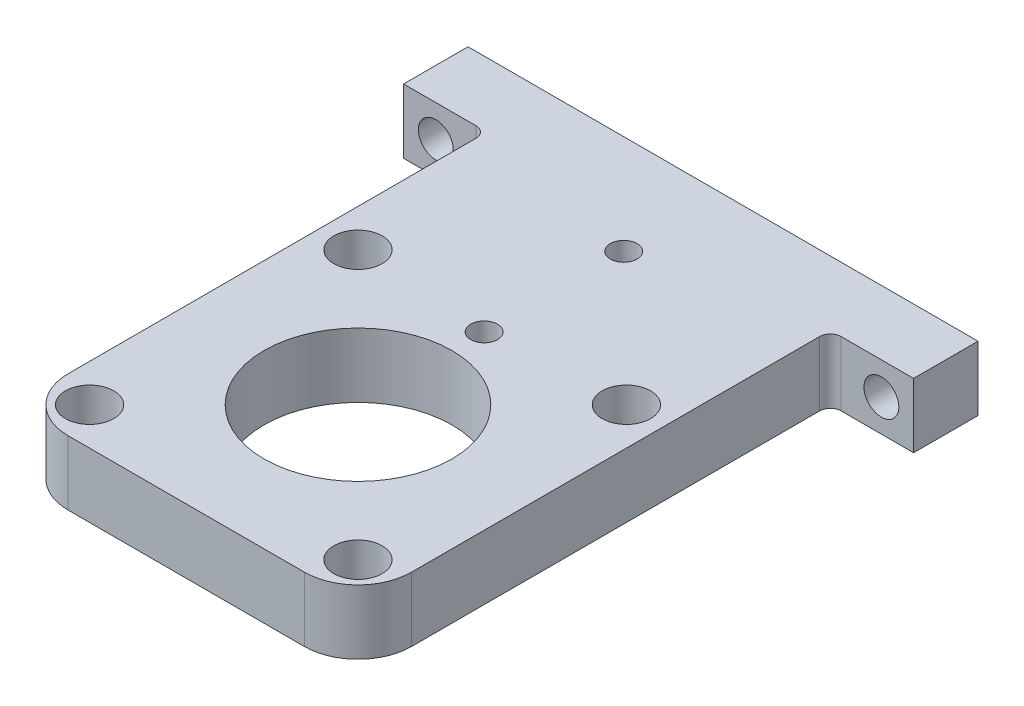
from build123d import *

# Parameters (mm, degrees)
SKETCH_1_W                = 95
SKETCH_1_H                = 100
EXTRUDE_1_DEPTH           = 12
SKETCH_9_W                = 15.5
SKETCH_9_H                = 88
CUT_EXTRUDE_4_DEPTH       = 139.452157802
HOLE_WIZARD_6_5_6_5_1_D   = 6.5
SKETCH_12_R               = 17.5
CUT_EXTRUDE_5_DEPTH       = 139.452157802
FILLET_1_R                = 10
HOLE_WIZARD_5_0_5_1_D     = 5
HOLE_WIZARD_5_0_5_1_DEPTH = 10
HOLE_WIZARD_5_0_5_1_TIP   = 1.502151548
FILLET_2_R                = 2
MM_1_D                    = 9
HOLE_WIZARD_M6_1_D        = 5
HOLE_WIZARD_M6_2_D        = 5


with BuildPart() as part:
    # 草图1 → 凸台-拉伸1 (new body)
    with BuildSketch(Plane(origin=(0, 0, 0), x_dir=(1, 0, 0), z_dir=(0, 1, 0))):
        with Locations((47.5, -50)):
            Rectangle(SKETCH_1_W, SKETCH_1_H)
    extrude(amount=EXTRUDE_1_DEPTH)

    # 草图9 → 切除-拉伸4 (cut, through all)
    with BuildSketch(Plane(origin=(0, 12, 0), x_dir=(1, 0, 0), z_dir=(0, 1, 0))):
        with Locations((7.75, -56)):
            Rectangle(SKETCH_9_W, SKETCH_9_H)
        with Locations((87.25, -56)):
            Rectangle(SKETCH_9_W, SKETCH_9_H)
    extrude(amount=-CUT_EXTRUDE_4_DEPTH, mode=Mode.SUBTRACT)

    # Ø6.5 (6.5) 直径孔1 (through all)
    with Locations(Plane.XY.offset(12)):
        with Locations((6, 6), (89, 6)):
            Hole(HOLE_WIZARD_6_5_6_5_1_D / 2)

    # 草图12 → 切除-拉伸5 (cut, through all)
    with BuildSketch(Plane(origin=(0, 12, 0), x_dir=(1, 0, 0), z_dir=(0, 1, 0))):
        with Locations(Location((47.5, -68, 0), (0, 0, 270))):
            Circle(SKETCH_12_R)
    extrude(amount=-CUT_EXTRUDE_5_DEPTH, mode=Mode.SUBTRACT)

    # 圆角1
    fillet_1_edges = [part.edges().sort_by_distance(p)[0] for p in [
        (15.5, 6, 100),
        (79.5, 6, 100),
    ]]
    fillet(fillet_1_edges, radius=FILLET_1_R)

    # Ø5.0 (5) 直径孔1
    with Locations(Plane(origin=(0, 0, 0), x_dir=(-1, 0, 0), z_dir=(0, 0, -1))):
        with Locations((-67.5, 6), (-27.5, 6)):
            Hole(HOLE_WIZARD_5_0_5_1_D / 2, depth=HOLE_WIZARD_5_0_5_1_DEPTH)
            with Locations((0, 0, -(HOLE_WIZARD_5_0_5_1_DEPTH + HOLE_WIZARD_5_0_5_1_TIP / 2))):  # 118° drill point
                Cone(0, HOLE_WIZARD_5_0_5_1_D / 2, HOLE_WIZARD_5_0_5_1_TIP, mode=Mode.SUBTRACT)

    # 圆角2
    fillet_2_edges = [part.edges().sort_by_distance(p)[0] for p in [
        (15.5, 6, 12),
        (79.5, 6, 12),
    ]]
    fillet(fillet_2_edges, radius=FILLET_2_R)

    # 大小mm 暗销孔1 (through all)
    with Locations(Plane(origin=(0, 0, 0), x_dir=(-1, 0, 0), z_dir=(0, -1, 0))):
        with Locations((-72.5, -43), (-72.5, -93), (-22.5, -93), (-22.5, -43)):
            Hole(MM_1_D / 2)

    # M6 螺纹孔1 (through all)
    with Locations(Plane(origin=(0, 0, 0), x_dir=(-1, 0, 0), z_dir=(0, -1, 0))):
        with Locations((-47.5, -44.5)):
            Hole(HOLE_WIZARD_M6_1_D / 2)

    # M6 螺纹孔2 (through all)
    with Locations(Plane(origin=(0, 0, 0), x_dir=(-1, 0, 0), z_dir=(0, -1, 0))):
        with Locations((-47.5, -18.5)):
            Hole(HOLE_WIZARD_M6_2_D / 2)


solid = part.part
